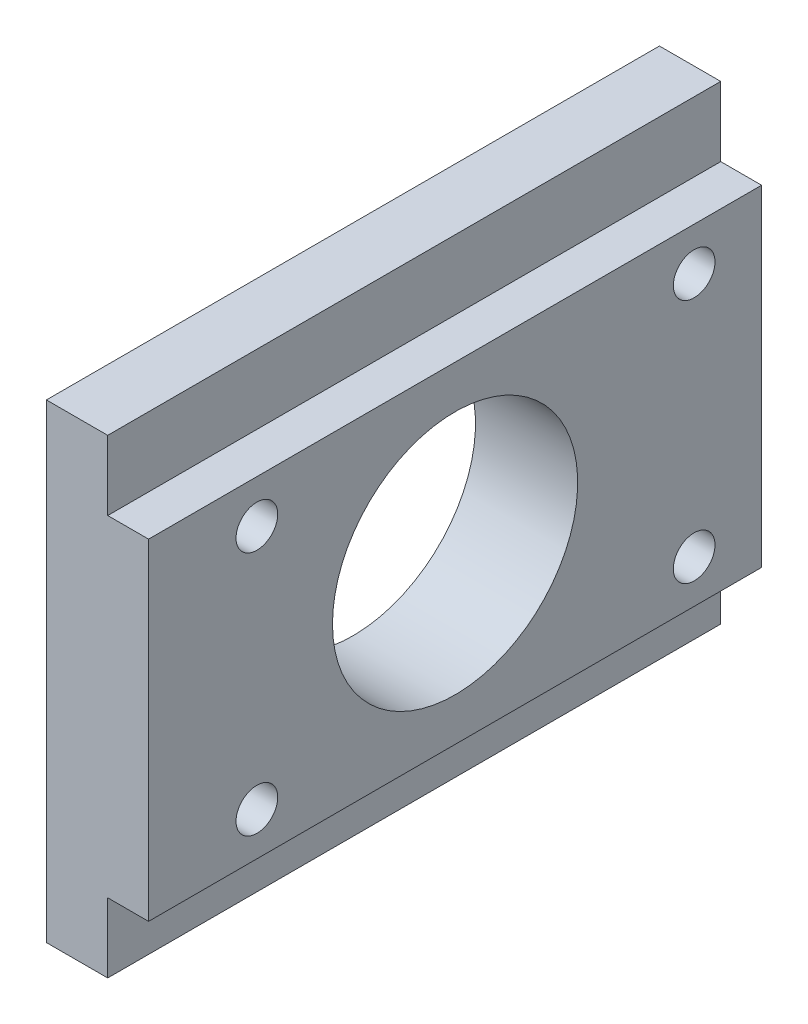
from build123d import *

# Parameters (mm, degrees)
EXTRUDE_1_DEPTH     = 75
SKETCH_2_R          = 30
CUT_EXTRUDE_1_DEPTH = 210
HOLE_WIZARD_M12_1_D = 10.2


with BuildPart() as part:
    # 草图1 → 凸台-拉伸1 (new, symmetric)
    with BuildSketch(Plane.XY):
        Polygon((0, 57.5), (0, -57.5), (15, -57.5), (15, -40.5), (25, -40.5), (25, 40.5), (15, 40.5), (15, 57.5), align=None)
    extrude(amount=EXTRUDE_1_DEPTH, both=True)

    # 草图2 → 切除-拉伸1 (cut)
    with BuildSketch(Plane.ZY):
        Circle(SKETCH_2_R)
    extrude(amount=-CUT_EXTRUDE_1_DEPTH, mode=Mode.SUBTRACT)

    # M12 螺纹孔1 (through all)
    with Locations(Plane.ZY):
        with Locations((-58.5, 30), (48.5, 30), (48.5, -30), (-58.5, -30)):
            Hole(HOLE_WIZARD_M12_1_D / 2)


solid = part.part
